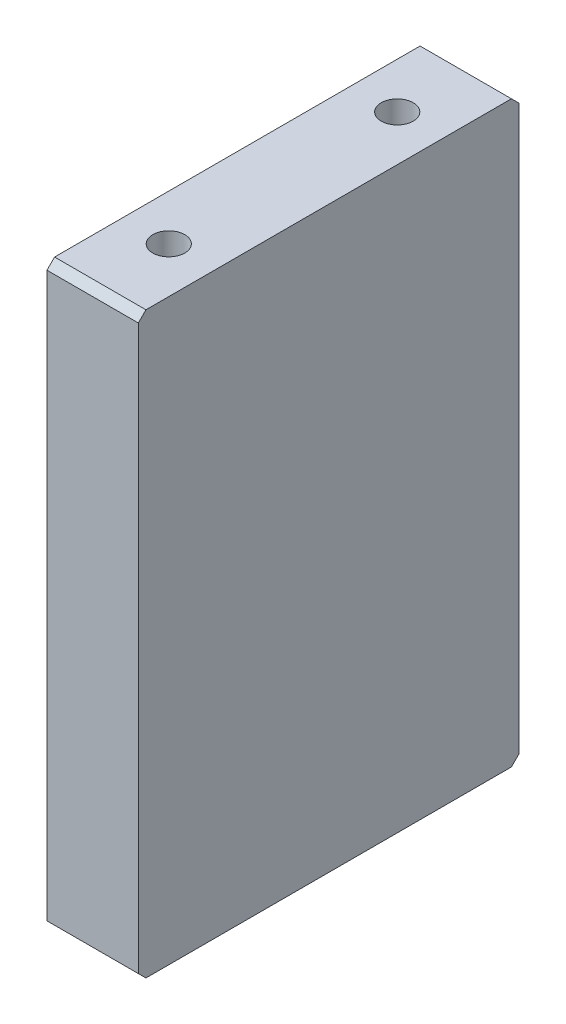
from build123d import *

# Parameters (mm, degrees)
SKETCH6_W                  = 50
SKETCH6_H                  = 76
BOSS_EXTRUDE6_DEPTH        = 12
M5_TAPPED_HOLE3_AT_2_COUNT = 2
M5_TAPPED_HOLE3_AT_2_PITCH = 30
CHAMFER1_SIZE              = 1


with BuildPart() as part:
    # Sketch6 → Boss-Extrude6 (new body)
    with BuildSketch(Plane(origin=(0, 0, 0), x_dir=(0, 0, -1), z_dir=(1, 0, 0))):
        with Locations((25, 0)):
            Rectangle(SKETCH6_W, SKETCH6_H)
    extrude(amount=-BOSS_EXTRUDE6_DEPTH)

    # Sketch19 → M5 Tapped Hole3 (revolve, cut)
    with BuildSketch(Plane(origin=(-6, -38, -10), x_dir=(0, 0, -1), z_dir=(1, 0, 0))):
        Polygon((0, 0), (0, 18.6618073), (2.1, 17.4), (2.1, 0), align=None)
    m5_tapped_hole3 = revolve(axis=Axis((-6, -44.35, -10), (0, 1, 0)), mode=Mode.SUBTRACT)

    # M5 Tapped Hole3 at 2: M5 Tapped Hole3 ×2
    with Locations(*[(0, 0, -i * M5_TAPPED_HOLE3_AT_2_PITCH) for i in range(1, M5_TAPPED_HOLE3_AT_2_COUNT)]):
        add(m5_tapped_hole3, mode=Mode.SUBTRACT)

    # Mirror1: M5 Tapped Hole3 across plane
    add(m5_tapped_hole3.mirror(Plane.ZX), mode=Mode.SUBTRACT)

    # Mirror1 copy 1 sketch → Mirror1 copy 1 (revolve, cut)
    with BuildSketch(Plane(origin=(-6, 38, -40), x_dir=(0, 0, -1), z_dir=(1, 0, 0))):
        Polygon((0, 0), (0, -18.6618073), (2.1, -17.4), (2.1, 0), align=None)
    revolve(axis=Axis((-6, 44.35, -40), (0, 1, 0)), mode=Mode.SUBTRACT)

    # Chamfer1
    chamfer1_edges = [part.edges().sort_by_distance(p)[0] for p in [
        (-6, 38, 0),
        (-6, 38, -50),
        (-6, -38, -50),
        (-6, -38, 0),
    ]]
    chamfer(chamfer1_edges, length=CHAMFER1_SIZE)


solid = part.part
